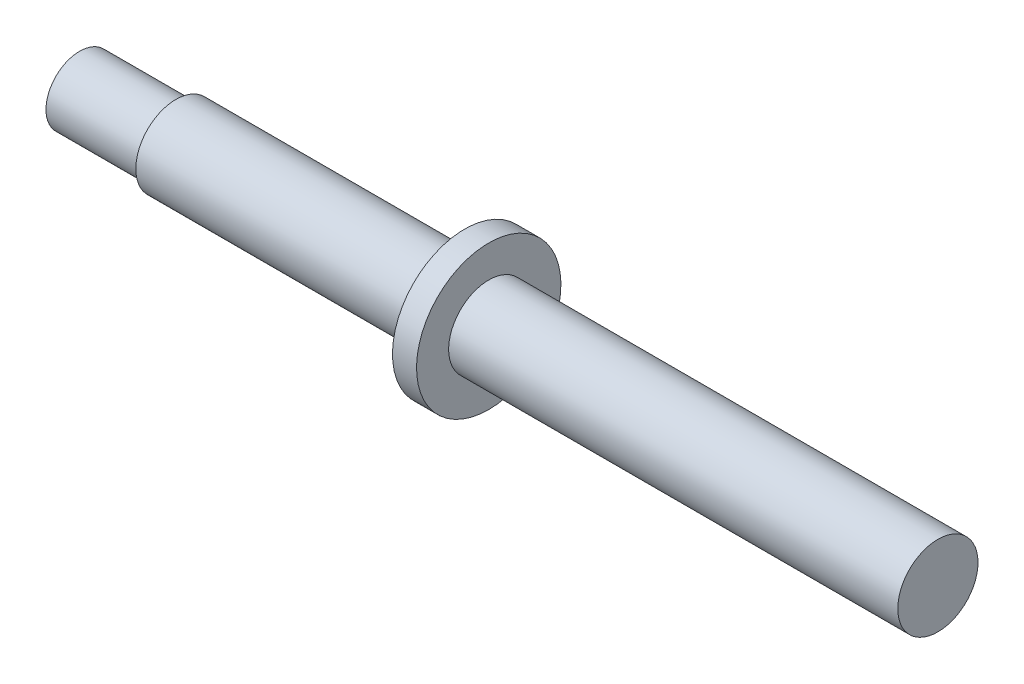
from build123d import *

# Parameters (mm, degrees)
BOSS_EXTRUDE_START   = 100
SKETCH_2_R           = 25
BOSS_EXTRUDE_1_DEPTH = 100
SKETCH_3_R           = 21
BOSS_EXTRUDE_2_DEPTH = 60


with BuildPart() as part:
    # Sketch 1 → Revolve 1 (revolve)
    with BuildSketch(Plane.XY, mode=Mode.PRIVATE) as revolve_1_sk:
        Polygon((-187.5, 0), (-187.5, 25), (-7.5, 25), (-7.5, 45), (7.5, 45), (7.5, 25), (187.5, 25), (187.5, 0), align=None)
    revolve(revolve_1_sk.sketch.rotate(Axis((-187.5, 0, 0), (1, 0, 0)), 180), axis=Axis((-187.5, 0, 0), (1, 0, 0)))

    # Sketch 2 → Boss-Extrude 1 (add)
    with BuildSketch(Plane(origin=(187.5, 0, 0), x_dir=(0, 0, -1), z_dir=(1, 0, 0)).offset(BOSS_EXTRUDE_START)):
        with Locations(Location((0, 0, 0), (0, 0, 270))):
            Circle(SKETCH_2_R)
    extrude(amount=-BOSS_EXTRUDE_1_DEPTH)

    # Sketch 3 → Boss-Extrude 2 (add)
    with BuildSketch(Plane.ZY.offset(187.5)):
        with Locations(Location((0, 0, 0), (0, 0, 270))):
            Circle(SKETCH_3_R)
    extrude(amount=BOSS_EXTRUDE_2_DEPTH)


solid = part.part
